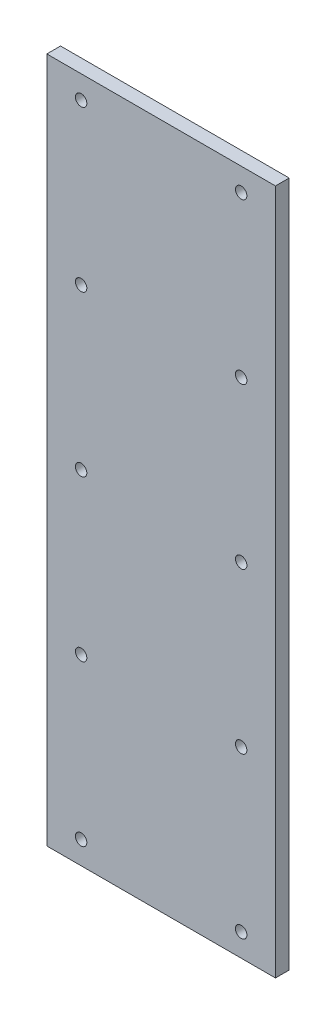
from build123d import *

# Parameters (mm, degrees)
SKETCH1_W            = 100
SKETCH1_H            = 300
BOSS_EXTRUDE1_DEPTH  = 6
M6_TAPPED_HOLE1_D    = 5
LPATTERN1_COUNT      = 3
LPATTERN1_PITCH      = 70
LPATTERN1_COUNT_DIR2 = 2
LPATTERN1_PITCH_DIR2 = 70
LPATTERN2_COUNT      = 3
LPATTERN2_PITCH      = 70
LPATTERN2_COPY_1_D   = 5
LPATTERN2_COPY_2_D   = 5
LPATTERN2_COPY_3_D   = 5
LPATTERN2_COPY_4_D   = 5
LPATTERN2_COPY_5_D   = 5
LPATTERN2_COPY_6_D   = 5
LPATTERN2_COPY_7_D   = 5
LPATTERN2_COPY_8_D   = 5
LPATTERN2_COPY_9_D   = 5
LPATTERN2_COPY_10_D  = 5


with BuildPart() as part:
    # Sketch1 → Boss-Extrude1 (new body)
    with BuildSketch(Plane.XY):
        Rectangle(SKETCH1_W, SKETCH1_H)
    extrude(amount=BOSS_EXTRUDE1_DEPTH)

    # M6 Tapped Hole1 (through all)
    with Locations(Plane.XY.offset(6)):
        with Locations((-35, 0)):
            m6_tapped_hole1 = Hole(M6_TAPPED_HOLE1_D / 2)

    # LPattern1: M6 Tapped Hole1 3 × 2
    with Locations(*[(j * LPATTERN1_PITCH_DIR2, -i * LPATTERN1_PITCH, 0) for i in range(LPATTERN1_COUNT) for j in range(LPATTERN1_COUNT_DIR2) if (i, j) != (0, 0)]):
        add(m6_tapped_hole1, mode=Mode.SUBTRACT)

    # LPattern2: M6 Tapped Hole1 ×3
    with Locations(*[(0, i * LPATTERN2_PITCH, 0) for i in range(1, LPATTERN2_COUNT)]):
        add(m6_tapped_hole1, mode=Mode.SUBTRACT)

    # LPattern2 copy 1 (through all)
    with Locations(Plane(origin=(70, 70, 6), x_dir=(1, 0, 0), z_dir=(0, 0, 1))):
        with Locations((-35, 0)):
            Hole(LPATTERN2_COPY_1_D / 2)

    # LPattern2 copy 2 (through all)
    with Locations(Plane(origin=(70, 140, 6), x_dir=(1, 0, 0), z_dir=(0, 0, 1))):
        with Locations((-35, 0)):
            Hole(LPATTERN2_COPY_2_D / 2)

    # LPattern2 copy 3 (through all)
    with Locations(Plane.XY.offset(6)):
        with Locations((-35, 0)):
            Hole(LPATTERN2_COPY_3_D / 2)

    # LPattern2 copy 4 (through all)
    with Locations(Plane(origin=(0, 70, 6), x_dir=(1, 0, 0), z_dir=(0, 0, 1))):
        with Locations((-35, 0)):
            Hole(LPATTERN2_COPY_4_D / 2)

    # LPattern2 copy 5 (through all)
    with Locations(Plane(origin=(70, 0, 6), x_dir=(1, 0, 0), z_dir=(0, 0, 1))):
        with Locations((-35, 0)):
            Hole(LPATTERN2_COPY_5_D / 2)

    # LPattern2 copy 6 (through all)
    with Locations(Plane(origin=(70, 70, 6), x_dir=(1, 0, 0), z_dir=(0, 0, 1))):
        with Locations((-35, 0)):
            Hole(LPATTERN2_COPY_6_D / 2)

    # LPattern2 copy 7 (through all)
    with Locations(Plane(origin=(0, -70, 6), x_dir=(1, 0, 0), z_dir=(0, 0, 1))):
        with Locations((-35, 0)):
            Hole(LPATTERN2_COPY_7_D / 2)

    # LPattern2 copy 8 (through all)
    with Locations(Plane.XY.offset(6)):
        with Locations((-35, 0)):
            Hole(LPATTERN2_COPY_8_D / 2)

    # LPattern2 copy 9 (through all)
    with Locations(Plane(origin=(70, -70, 6), x_dir=(1, 0, 0), z_dir=(0, 0, 1))):
        with Locations((-35, 0)):
            Hole(LPATTERN2_COPY_9_D / 2)

    # LPattern2 copy 10 (through all)
    with Locations(Plane(origin=(70, 0, 6), x_dir=(1, 0, 0), z_dir=(0, 0, 1))):
        with Locations((-35, 0)):
            Hole(LPATTERN2_COPY_10_D / 2)


solid = part.part
